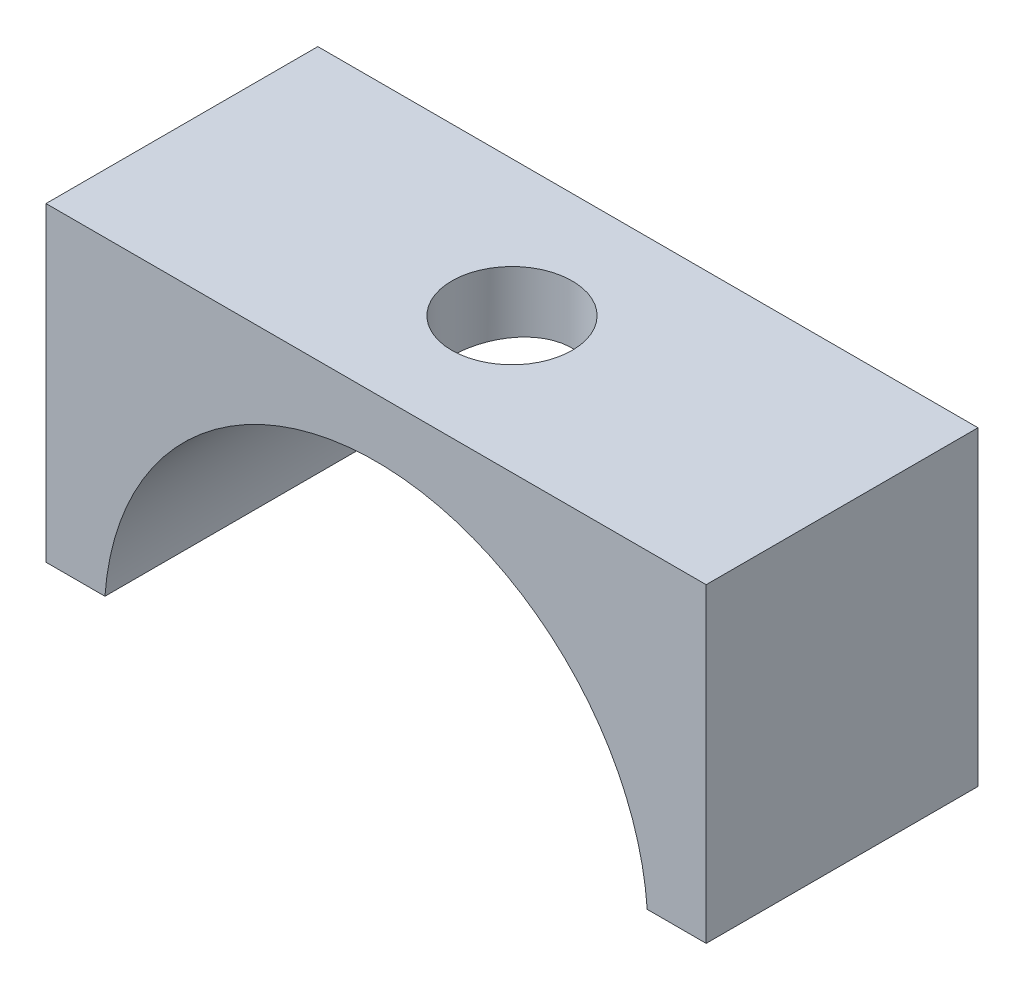
from build123d import *

# Parameters (mm, degrees)
EXTRUDE_1_DEPTH     = 7
SKETCH_2_R          = 1.55
CUT_EXTRUDE_1_DEPTH = 7


with BuildPart() as part:
    # 草图1 → 凸台-拉伸1 (new body)
    with BuildSketch(Plane.XY):
        with BuildLine():
            Line((8.5, 8.5), (-8.5, 8.5))
            Line((-8.5, 8.5), (-8.5, 0.5))
            Line((-8.5, 0.5), (-6.982120022, 0.5))
            ThreePointArc((-6.982120022, 0.5), (0, 7), (6.982120022, 0.5))
            Line((6.982120022, 0.5), (8.5, 0.5))
            Line((8.5, 0.5), (8.5, 8.5))
        make_face()
    extrude(amount=EXTRUDE_1_DEPTH)

    # 草图2 → 切除-拉伸1 (cut)
    with BuildSketch(Plane(origin=(0, 8.5, 0), x_dir=(1, 0, 0), z_dir=(0, 1, 0))):
        with Locations(Location((0, -3.5, 0), (0, 0, 270))):
            Circle(SKETCH_2_R)
    extrude(amount=-CUT_EXTRUDE_1_DEPTH, mode=Mode.SUBTRACT)


solid = part.part
